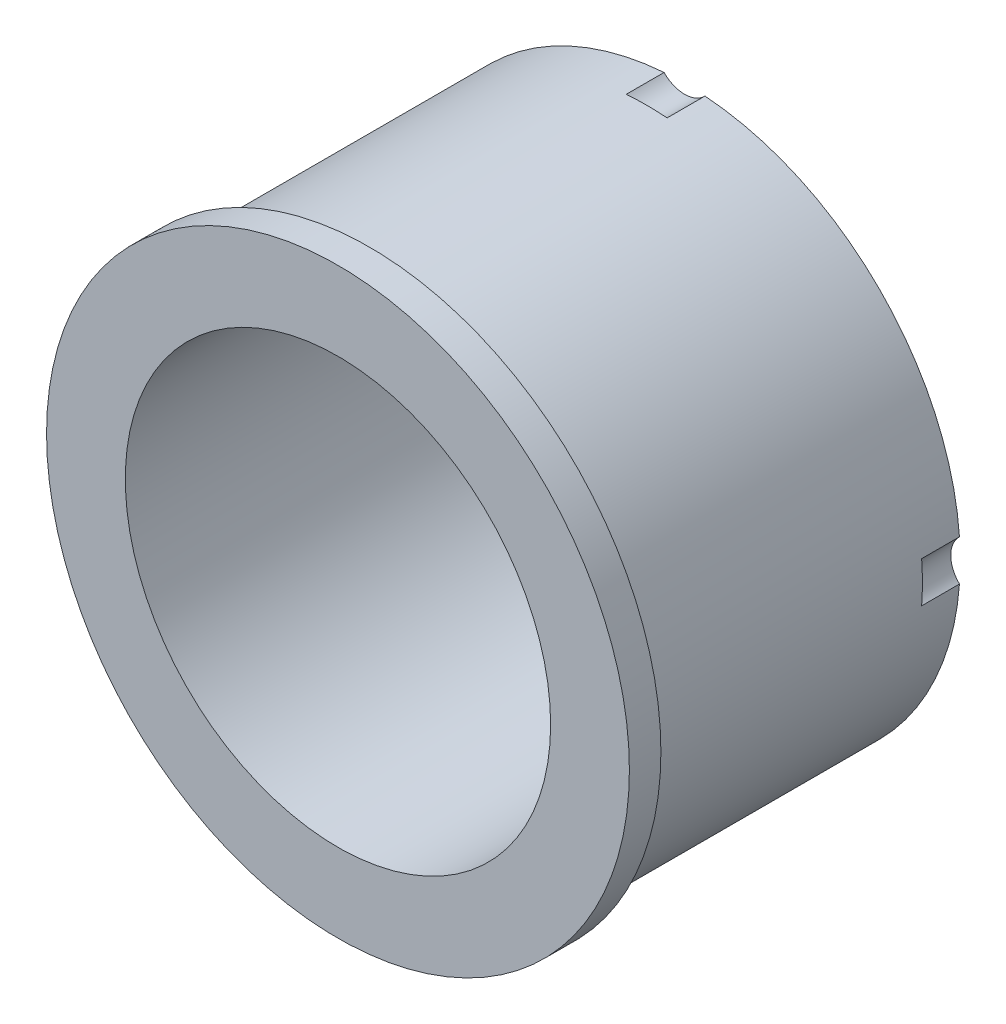
from build123d import *

# Parameters (mm, degrees)
SKETCH1_W           = 92.5
SKETCH1_H           = 10
SKETCH2_R           = 87.5
BOSS_EXTRUDE1_DEPTH = 100
CUT_EXTRUDE1_START  = -12
CUT_EXTRUDE1_DEPTH  = 12
CUT_EXTRUDE2_START  = -12
CUT_EXTRUDE2_DEPTH  = 12
CUT_EXTRUDE3_START  = -12
CUT_EXTRUDE3_DEPTH  = 12
CUT_EXTRUDE4_START  = -12
CUT_EXTRUDE4_DEPTH  = 12
HOLE1_D             = 135


with BuildPart() as part:
    # Sketch1 → Revolve1 (revolve)
    with BuildSketch(Plane(origin=(0, 234.743963655, 0), x_dir=(1, 0, 0), z_dir=(0, 1, 0))):
        with Locations((567.480642584, 1252.692981355)):
            Rectangle(SKETCH1_W, SKETCH1_H)
    revolve(axis=Axis((521.230642584, 234.743963655, -1257.692981355), (0, 0, 1)))

    # Sketch2 → Boss-Extrude1 (add)
    with BuildSketch(Plane(origin=(0, 0, -1257.692981355), x_dir=(-1, 0, 0), z_dir=(0, 0, -1))):
        with Locations((-521.230642584, 234.743963655)):
            Circle(SKETCH2_R)
    extrude(amount=BOSS_EXTRUDE1_DEPTH)

    # Sketch3 → Cut-Extrude1 (cut)
    with BuildSketch(Plane(origin=(0, 0, -1357.692981355), x_dir=(-1, 0, 0), z_dir=(0, 0, -1)).offset(CUT_EXTRUDE1_START)):
        with BuildLine():
            ThreePointArc((-433.971284296, 241.228899354), (-436.730642584, 234.743963655), (-433.971284296, 228.259027955))
            ThreePointArc((-433.971284296, 228.259027955), (-433.730642584, 234.743963655), (-433.971284296, 241.228899354))
        make_face()
    extrude(amount=CUT_EXTRUDE1_DEPTH, mode=Mode.SUBTRACT)

    # Sketch4 → Cut-Extrude2 (cut)
    with BuildSketch(Plane(origin=(0, 0, -1357.692981355), x_dir=(-1, 0, 0), z_dir=(0, 0, -1)).offset(CUT_EXTRUDE2_START)):
        with BuildLine():
            ThreePointArc((-514.745706884, 147.484605366), (-521.230642584, 150.243963655), (-527.715578284, 147.484605366))
            ThreePointArc((-527.715578284, 147.484605366), (-521.230642584, 147.243963655), (-514.745706884, 147.484605366))
        make_face()
    extrude(amount=CUT_EXTRUDE2_DEPTH, mode=Mode.SUBTRACT)

    # Sketch5 → Cut-Extrude3 (cut)
    with BuildSketch(Plane(origin=(0, 0, -1357.692981355), x_dir=(-1, 0, 0), z_dir=(0, 0, -1)).offset(CUT_EXTRUDE3_START)):
        with BuildLine():
            ThreePointArc((-527.715578284, 322.003321943), (-521.230642584, 319.243963655), (-514.745706884, 322.003321943))
            ThreePointArc((-514.745706884, 322.003321943), (-521.230642584, 322.243963655), (-527.715578284, 322.003321943))
        make_face()
    extrude(amount=CUT_EXTRUDE3_DEPTH, mode=Mode.SUBTRACT)

    # Sketch6 → Cut-Extrude4 (cut)
    with BuildSketch(Plane(origin=(0, 0, -1357.692981355), x_dir=(-1, 0, 0), z_dir=(0, 0, -1)).offset(CUT_EXTRUDE4_START)):
        with BuildLine():
            ThreePointArc((-608.490000873, 228.259027955), (-605.730642584, 234.743963654), (-608.490000873, 241.228899354))
            ThreePointArc((-608.490000873, 241.228899354), (-608.730642584, 234.743963654), (-608.490000873, 228.259027955))
        make_face()
    extrude(amount=CUT_EXTRUDE4_DEPTH, mode=Mode.SUBTRACT)

    # Hole1 (through all)
    with Locations(Plane.XY.offset(-1247.692981355)):
        with Locations((521.230642584, 234.743963655)):
            Hole(HOLE1_D / 2)


solid = part.part
